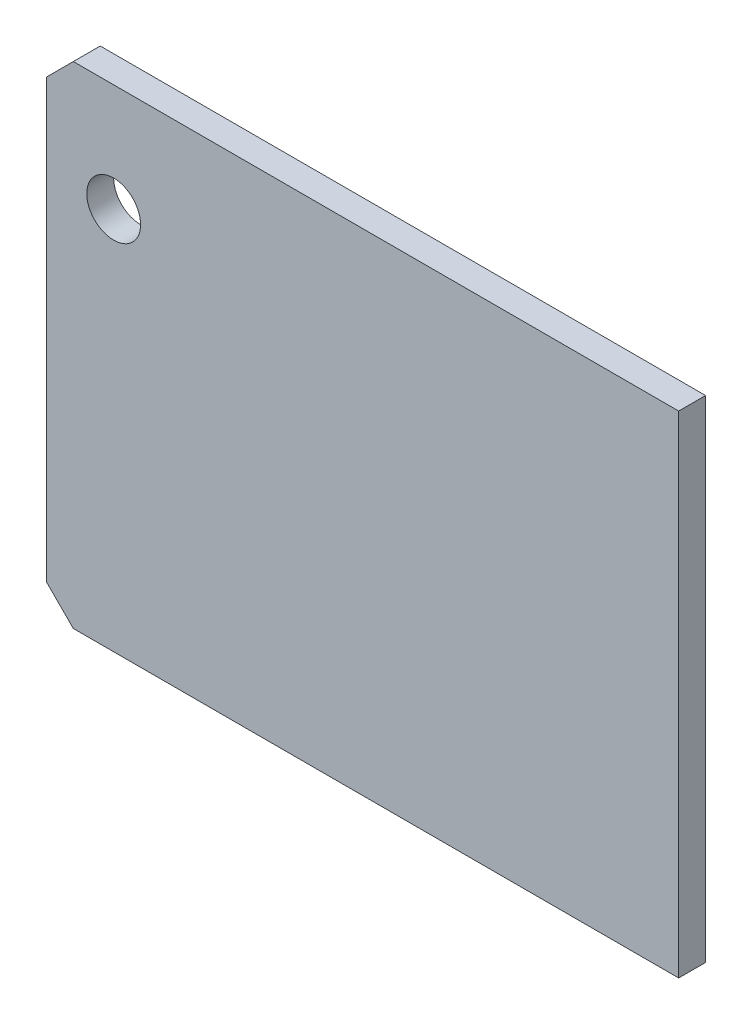
SolidWorks part; units mm, degrees
ref_plane "Front Plane" through (0, 0, 0) normal (0, 0, 1) x (1, 0, 0)
ref_plane "Top Plane" through (0, 0, 0) normal (0, 1, 0) x (1, 0, 0)
ref_plane "Right Plane" through (0, 0, 0) normal (1, 0, 0) x (0, 0, -1)
sketch "Sketch1" plane through (0, 0, 0) normal (0, 0, 1) x (1, 0, 0)
  line L1 (235, 182.5) -> (-235, 182.5)
  line L2 (235, 182.5) -> (235, -182.5)
  line L3 (235, -182.5) -> (-235, -182.5)
  line L4 (-235, 182.5) -> (-235, -182.5)
  line L5 (235, 182.5) -> (-235, -182.5) construction
  line L6 (235, -182.5) -> (-235, 182.5) construction
  point P0 (0, 0)
  dimension "D1" = 470
  dimension "D2" = 365
extrude "Boss-Extrude1" add sketch "Sketch1" along normal blind 20
chamfer "Chamfer1" distance 20 angle 45 1 edges at (-235, 182.5, 10)
sketch "Sketch2" plane through (0, 0, 20) normal (0, 0, 1) x (1, 0, 0)
  line L0 (-235, 162.5) -> (-235, -182.5) construction
  line L1 (235, 182.5) -> (-215, 182.5) construction
  circle A0 centre (-185, 102.5) radius 20
  dimension "D3" = 40
  dimension "D1" = 50
  dimension "D2" = 80
extrude "Cut-Extrude1" cut sketch "Sketch2" against normal through all both and the other way through all
chamfer "Chamfer2" distance 20 angle 45 1 edges at (-235, -182.5, 10)
